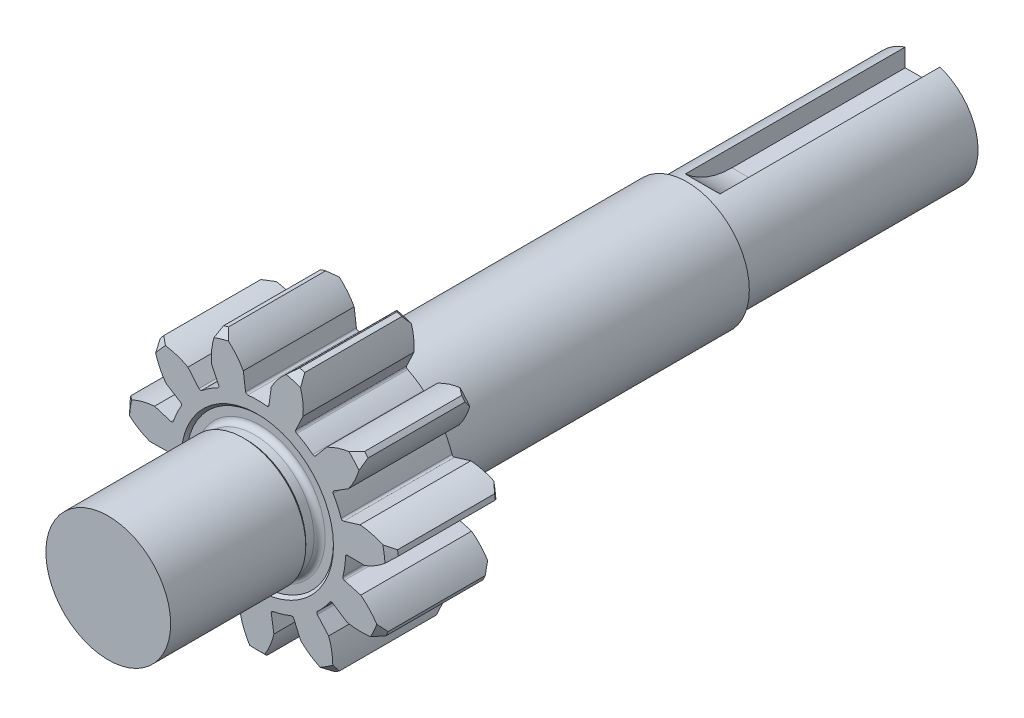
SolidWorks part; units mm, degrees
ref_plane "Middle plane" through (0, 0, 0) normal (0, 0, 1) x (1, 0, 0)
ref_plane "Top Plane" through (0, 0, 0) normal (0, 1, 0) x (1, 0, 0)
ref_plane "Right Plane" through (0, 0, 0) normal (1, 0, 0) x (0, 0, -1)
sketch "Spur gear" plane through (0, 0, 0) normal (0, 0, 1) x (1, 0, 0)
  line L0 (0, 0) -> (-2.3482, 16.3321) construction
  line L2 (-2.0154, 15.3734) -> (0, 0)
  line L3 (0, 0) -> (0, 52) construction
  line L4 (2.3482, 16.3321) -> (0, 0) construction
  line L6 (0, 0) -> (2.0154, 15.3734)
  circle A0 centre (0, 0) radius 15.5049
  circle A1 centre (0, 0) radius 12.75
  arc A2 (2.3482, 16.3321) -> (-2.3482, 16.3321) centre (0, 0) ccw
  circle A3 centre (0, 0) radius 19.5
  spline S0 degree 4 poles (0.7936, 14.8906) (0.7924, 14.9201) (0.7881, 14.9788) (0.7725, 15.0958) (0.7289, 15.316) (0.6484, 15.6067) (0.4539, 16.1447) (0.0492, 16.9597) (-0.6377, 17.9757) (-1.7913, 19.243) (-3.3499, 20.5096) (-5.2443, 21.6406) (-7.4338, 22.5657) (-9.7197, 23.2127) (-12.0632, 23.5974) (-14.5507, 23.7418) (-17.633, 23.5986) (-21.2621, 22.9576) (-25.3266, 21.6048) (-29.5547, 19.4226) (-33.4233, 16.6565) (-36.4497, 13.8025) (-38.7654, 11.0977) (-40.5023, 8.6952) (-41.7738, 6.6932) (-43.2134, 4.102) (-44.4514, 1.4058) (-45.4859, -1.3736) (-46.4831, -4.7889) (-47.0485, -7.396) (-47.4104, -9.7431) (-47.6077, -11.655) (-47.6802, -12.5487) (-47.7381, -13.4181) (-47.7759, -14.2391) (-47.8017, -14.99) (-47.8125, -16.0362) (-47.809, -16.7047) (-47.7875, -17.792) (-47.7473, -18.6332) (-47.688, -19.6577) (-47.6107, -20.5673) (-47.515, -21.548) (-47.4014, -22.4756) (-47.3026, -23.2033) (-47.2309, -23.6656) (-47.1936, -23.9061) knots 0 0 0 0 0 0.001401 0.002802 0.005604 0.010661 0.015718 0.02996 0.048734 0.068727 0.096889 0.125051 0.153212 0.181374 0.209535 0.237696 0.271429 0.327752 0.384075 0.440398 0.496721 0.553044 0.581206 0.609367 0.637529 0.66569 0.722013 0.750174 0.778336 0.834659 0.84874 0.86282 0.869861 0.876901 0.890982 0.900036 0.909091 0.920455 0.931818 0.943182 0.954545 0.965909 0.977273 0.988636 1 1 1 1 1 construction
  spline S1 degree 4 poles (-2.0154, 15.3734) (-2.1011, 15.5352) (-2.3813, 16.0225) (-2.9403, 16.8122) (-3.9842, 17.9417) (-5.4871, 19.1443) (-7.3108, 20.2145) (-9.4159, 21.0852) (-11.6114, 21.6888) (-13.8601, 22.0406) (-16.2451, 22.1609) (-19.1981, 22.0014) (-22.6715, 21.3607) (-26.557, 20.0349) (-30.5934, 17.9129) (-34.281, 15.2339) (-37.1607, 12.4768) (-39.3605, 9.8678) (-41.0077, 7.5528) (-42.2118, 5.6248) (-43.5728, 3.1311) (-44.7397, 0.5381) (-45.711, -2.1331) (-46.642, -5.4134) (-47.1651, -7.9161) (-47.4949, -10.1682) (-47.6701, -12.0019) (-47.7331, -12.8589) (-47.7823, -13.6926) (-47.8127, -14.4797) (-47.8319, -15.1995) (-47.8347, -16.2022) (-47.8265, -16.8429) (-47.798, -17.8848) (-47.7547, -18.6666) (-47.709, -19.3683) (-47.6743, -19.799) (-47.6569, -19.9982) knots 0.020881 0.020881 0.020881 0.020881 0.020881 0.02996 0.048734 0.068727 0.096889 0.125051 0.153212 0.181374 0.209535 0.237696 0.271429 0.327752 0.384075 0.440398 0.496721 0.553044 0.581206 0.609367 0.637529 0.66569 0.722013 0.750174 0.778336 0.834659 0.84874 0.86282 0.869861 0.876901 0.890982 0.900036 0.909091 0.920455 0.931818 0.943182 0.953189 0.953189 0.953189 0.953189 0.953189
  spline S2 degree 4 poles (-0.7936, 14.8906) (-0.7924, 14.9201) (-0.7881, 14.9788) (-0.7725, 15.0958) (-0.7289, 15.316) (-0.6484, 15.6067) (-0.4539, 16.1447) (-0.0492, 16.9597) (0.6377, 17.9757) (1.7913, 19.243) (3.3499, 20.5096) (5.2443, 21.6406) (7.4338, 22.5657) (9.7197, 23.2127) (12.0632, 23.5974) (14.5507, 23.7418) (17.633, 23.5986) (21.2621, 22.9576) (25.3266, 21.6048) (29.5547, 19.4226) (33.4233, 16.6565) (36.4497, 13.8025) (38.7654, 11.0977) (40.5023, 8.6952) (41.7738, 6.6932) (43.2134, 4.102) (44.4514, 1.4058) (45.4859, -1.3736) (46.4831, -4.7889) (47.0485, -7.396) (47.4104, -9.7431) (47.6077, -11.655) (47.6802, -12.5487) (47.7381, -13.4181) (47.7759, -14.2391) (47.8017, -14.99) (47.8125, -16.0362) (47.809, -16.7047) (47.7875, -17.792) (47.7473, -18.6332) (47.688, -19.6577) (47.6107, -20.5673) (47.515, -21.548) (47.4014, -22.4756) (47.3026, -23.2033) (47.2309, -23.6656) (47.1936, -23.9061) knots 0 0 0 0 0 0.001401 0.002802 0.005604 0.010661 0.015718 0.02996 0.048734 0.068727 0.096889 0.125051 0.153212 0.181374 0.209535 0.237696 0.271429 0.327752 0.384075 0.440398 0.496721 0.553044 0.581206 0.609367 0.637529 0.66569 0.722013 0.750174 0.778336 0.834659 0.84874 0.86282 0.869861 0.876901 0.890982 0.900036 0.909091 0.920455 0.931818 0.943182 0.954545 0.965909 0.977273 0.988636 1 1 1 1 1 construction
  spline S3 degree 4 poles (2.0154, 15.3734) (2.1011, 15.5352) (2.3813, 16.0225) (2.9403, 16.8122) (3.9842, 17.9417) (5.4871, 19.1443) (7.3108, 20.2145) (9.4159, 21.0852) (11.6114, 21.6888) (13.8601, 22.0406) (16.2451, 22.1609) (19.1981, 22.0014) (22.6715, 21.3607) (26.557, 20.0349) (30.5934, 17.9129) (34.281, 15.2339) (37.1607, 12.4768) (39.3605, 9.8678) (41.0077, 7.5528) (42.2118, 5.6248) (43.5728, 3.1311) (44.7397, 0.5381) (45.711, -2.1331) (46.642, -5.4134) (47.1651, -7.9161) (47.4949, -10.1682) (47.6701, -12.0019) (47.7331, -12.8589) (47.7823, -13.6926) (47.8127, -14.4797) (47.8319, -15.1995) (47.8347, -16.2022) (47.8265, -16.8429) (47.798, -17.8848) (47.7547, -18.6666) (47.709, -19.3683) (47.6743, -19.799) (47.6569, -19.9982) knots 0.020881 0.020881 0.020881 0.020881 0.020881 0.02996 0.048734 0.068727 0.096889 0.125051 0.153212 0.181374 0.209535 0.237696 0.271429 0.327752 0.384075 0.440398 0.496721 0.553044 0.581206 0.609367 0.637529 0.66569 0.722013 0.750174 0.778336 0.834659 0.84874 0.86282 0.869861 0.876901 0.890982 0.900036 0.909091 0.920455 0.931818 0.943182 0.953189 0.953189 0.953189 0.953189 0.953189
sketch "Circle" plane through (0, 0, 0) normal (0, 0, 1) x (1, 0, 0)
  circle A0 centre (0, 0) radius 19.5 construction
  circle A1 centre (0, 0) radius 19.5
extrude "Blank" add sketch "Circle" along normal mid plane 16
chamfer "Tooth chamfer" distance 1 angle 45 2 edges at (19.5, 0, -8) (19.5, 0, 8)
sketch "Tooth profile" plane through (0, 0, 0) normal (0, 0, 1) x (1, 0, 0)
  line L4 (0, 0) -> (2.0154, 15.3734) construction
  line L5 (-2.0154, 15.3734) -> (0, 0) construction
  line L6 (0, 0) -> (2.0154, 15.3734)
  line L7 (-2.0154, 15.3734) -> (0, 0)
  circle A4 centre (0, 0) radius 12.75 construction
  circle A5 centre (0, 0) radius 19.5 construction
  circle A6 centre (0, 0) radius 12.75
  circle A7 centre (0, 0) radius 19.5
  spline S1 degree 4 poles (999.7609, -51.6744) (36.065, -17.0379) (-0.5755, 0.4417) (-1.8205, 11.6607) (3.9842, 17.9417) (5.4871, 19.1443) (7.3108, 20.2145) (9.4159, 21.0852) (11.6114, 21.6888) (13.8601, 22.0406) (16.2451, 22.1609) (19.1981, 22.0014) (22.6715, 21.3607) (26.557, 20.0349) (30.5934, 17.9129) (34.281, 15.2339) (37.1607, 12.4768) (39.3605, 9.8678) (41.0077, 7.5528) (42.2118, 5.6248) (43.5728, 3.1311) (44.7397, 0.5381) (45.711, -2.1331) (46.642, -5.4134) (47.1651, -7.9161) (47.4949, -10.1682) (47.6701, -12.0019) (47.7331, -12.8589) (47.7823, -13.6926) (47.8127, -14.4797) (47.8319, -15.1995) (47.8347, -16.2022) (47.8265, -16.8429) (47.798, -17.8848) (47.5897, -21.6461) (46.8818, -29.7714) (46.3891, 13.6269) (33.8189, -1019.6941) knots -0.325788 -0.325788 -0.325788 -0.325788 -0.325788 0.02996 0.048734 0.068727 0.096889 0.125051 0.153212 0.181374 0.209535 0.237696 0.271429 0.327752 0.384075 0.440398 0.496721 0.553044 0.581206 0.609367 0.637529 0.66569 0.722013 0.750174 0.778336 0.834659 0.84874 0.86282 0.869861 0.876901 0.890982 0.900036 0.909091 0.920455 0.931818 0.943182 1.121242 1.121242 1.121242 1.121242 1.121242 only from (2.0154, 15.3734) to (47.6569, -19.9982) construction
  spline S3 degree 4 poles (-999.7609, -51.6744) (-36.065, -17.0379) (0.5755, 0.4417) (1.8205, 11.6607) (-3.9842, 17.9417) (-5.4871, 19.1443) (-7.3108, 20.2145) (-9.4159, 21.0852) (-11.6114, 21.6888) (-13.8601, 22.0406) (-16.2451, 22.1609) (-19.1981, 22.0014) (-22.6715, 21.3607) (-26.557, 20.0349) (-30.5934, 17.9129) (-34.281, 15.2339) (-37.1607, 12.4768) (-39.3605, 9.8678) (-41.0077, 7.5528) (-42.2118, 5.6248) (-43.5728, 3.1311) (-44.7397, 0.5381) (-45.711, -2.1331) (-46.642, -5.4134) (-47.1651, -7.9161) (-47.4949, -10.1682) (-47.6701, -12.0019) (-47.7331, -12.8589) (-47.7823, -13.6926) (-47.8127, -14.4797) (-47.8319, -15.1995) (-47.8347, -16.2022) (-47.8265, -16.8429) (-47.798, -17.8848) (-47.5897, -21.6461) (-46.8818, -29.7714) (-46.3891, 13.6269) (-33.8189, -1019.6941) knots -0.325788 -0.325788 -0.325788 -0.325788 -0.325788 0.02996 0.048734 0.068727 0.096889 0.125051 0.153212 0.181374 0.209535 0.237696 0.271429 0.327752 0.384075 0.440398 0.496721 0.553044 0.581206 0.609367 0.637529 0.66569 0.722013 0.750174 0.778336 0.834659 0.84874 0.86282 0.869861 0.876901 0.890982 0.900036 0.909091 0.920455 0.931818 0.943182 1.121242 1.121242 1.121242 1.121242 1.121242 only from (-2.0154, 15.3734) to (-47.6569, -19.9982) construction
  spline S4 degree 4 poles (2.0154, 15.3734) (2.1011, 15.5352) (2.3813, 16.0225) (2.9403, 16.8122) (3.9842, 17.9417) (5.4871, 19.1443) (7.3108, 20.2145) (9.4159, 21.0852) (11.6114, 21.6888) (13.8601, 22.0406) (16.2451, 22.1609) (19.1981, 22.0014) (22.6715, 21.3607) (26.557, 20.0349) (30.5934, 17.9129) (34.281, 15.2339) (37.1607, 12.4768) (39.3605, 9.8678) (41.0077, 7.5528) (42.2118, 5.6248) (43.5728, 3.1311) (44.7397, 0.5381) (45.711, -2.1331) (46.642, -5.4134) (47.1651, -7.9161) (47.4949, -10.1682) (47.6701, -12.0019) (47.7331, -12.8589) (47.7823, -13.6926) (47.8127, -14.4797) (47.8319, -15.1995) (47.8347, -16.2022) (47.8265, -16.8429) (47.798, -17.8848) (47.7547, -18.6666) (47.709, -19.3683) (47.6743, -19.799) (47.6569, -19.9982) knots 0.020881 0.020881 0.020881 0.020881 0.020881 0.02996 0.048734 0.068727 0.096889 0.125051 0.153212 0.181374 0.209535 0.237696 0.271429 0.327752 0.384075 0.440398 0.496721 0.553044 0.581206 0.609367 0.637529 0.66569 0.722013 0.750174 0.778336 0.834659 0.84874 0.86282 0.869861 0.876901 0.890982 0.900036 0.909091 0.920455 0.931818 0.943182 0.953189 0.953189 0.953189 0.953189 0.953189
  spline S5 degree 4 poles (-2.0154, 15.3734) (-2.1011, 15.5352) (-2.3813, 16.0225) (-2.9403, 16.8122) (-3.9842, 17.9417) (-5.4871, 19.1443) (-7.3108, 20.2145) (-9.4159, 21.0852) (-11.6114, 21.6888) (-13.8601, 22.0406) (-16.2451, 22.1609) (-19.1981, 22.0014) (-22.6715, 21.3607) (-26.557, 20.0349) (-30.5934, 17.9129) (-34.281, 15.2339) (-37.1607, 12.4768) (-39.3605, 9.8678) (-41.0077, 7.5528) (-42.2118, 5.6248) (-43.5728, 3.1311) (-44.7397, 0.5381) (-45.711, -2.1331) (-46.642, -5.4134) (-47.1651, -7.9161) (-47.4949, -10.1682) (-47.6701, -12.0019) (-47.7331, -12.8589) (-47.7823, -13.6926) (-47.8127, -14.4797) (-47.8319, -15.1995) (-47.8347, -16.2022) (-47.8265, -16.8429) (-47.798, -17.8848) (-47.7547, -18.6666) (-47.709, -19.3683) (-47.6743, -19.799) (-47.6569, -19.9982) knots 0.020881 0.020881 0.020881 0.020881 0.020881 0.02996 0.048734 0.068727 0.096889 0.125051 0.153212 0.181374 0.209535 0.237696 0.271429 0.327752 0.384075 0.440398 0.496721 0.553044 0.581206 0.609367 0.637529 0.66569 0.722013 0.750174 0.778336 0.834659 0.84874 0.86282 0.869861 0.876901 0.890982 0.900036 0.909091 0.920455 0.931818 0.943182 0.953189 0.953189 0.953189 0.953189 0.953189
extrude "Gear shaping" cut sketch "Tooth profile" against normal mid plane 16 contours S5 A6 S4 A7
fillet "Fillet1" [suppressed] radius 0.3
pattern_circular "CirPattern1" [suppressed] count 11 over 360
fillet "Fillet2" radius 0.3 2 edges at (1.6573, 12.6418, 0) (-1.6573, 12.6418, 0)
pattern_circular "CirPattern2" count 11 over 360 about axis through (0, 0, 8) along (0, 0, -1) of "Fillet2", "Gear shaping"
sketch "Pitch circle" plane through (0, 0, 0) normal (0, 0, 1) x (1, 0, 0)
  circle A0 centre (0, 0) radius 16.5 construction
  circle A1 centre (0, 0) radius 16.5 construction
sketch "Sketch1" plane through (0, 0, 8) normal (0, 0, 1) x (1, 0, 0)
  circle A0 centre (0, 0) radius 9
  dimension "D1" = 18
extrude "Boss-Extrude1" add sketch "Sketch1" along normal blind 21.5
sketch "Sketch2" plane through (0, 0, 29.5) normal (0, 0, 1) x (1, 0, 0)
  circle A0 centre (0, 0) radius 8
  dimension "D1" = 16
extrude "Boss-Extrude2" add sketch "Sketch2" along normal blind 34 from offset 117.5 separate body offset against normal yes
sketch "Sketch3" plane through (0, 0, -54) normal (0, 0, 1) x (1, 0, 0)
  circle A0 centre (0, 0) radius 9
  dimension "D1" = 18
extrude "Boss-Extrude3" add sketch "Sketch3" along normal up to surface (46 mm away) up to face at (0, 0, -8)
sketch "Sketch4" plane through (0, 0, 0) normal (1, 0, 0) x (0, 0, -1)
  line L0 (88, 5) -> (63, 5)
  line L1 (88, -8) -> (88, 8) construction
  line L2 (55.8586, 8) -> (88, 8)
  line L3 (88, 8) -> (88, 5)
  line L4 (54, -8) -> (88, -8) construction
  arc A0 (63, 5) -> (55.8586, 8) centre (63, 15) cw
  dimension "D1" = 25
  dimension "D2" = 10
  dimension "D3" = 25
  dimension "D4" = 13
extrude "Cut-Extrude1" cut sketch "Sketch4" against normal mid plane 5
sketch "Sketch5" plane through (0, 0, 0) normal (1, 0, 0) x (0, 0, -1)
  line L4 (8, 11) -> (7.6, 10.6)
  line L5 (8, 9) -> (7.6, 8.6) construction
  line L6 (8, 9) -> (10, 9)
  line L7 (7.6, 8.6) -> (9.6, 8.6)
  line L8 (10, 9) -> (9.6, 8.6)
  line L9 (7.6, 8.6) -> (7.6, 10.6)
  line L10 (8, 9) -> (8, 11)
  line L11 (0, 0) -> (0, 9.5985) construction
  line L12 (0, 16.5) -> (0, -16.5) construction
  line L14 (-8, 9) -> (-7.6, 8.6) construction
  line L15 (-8, 9) -> (-8, 11)
  line L16 (-7.6, 8.6) -> (-7.6, 10.6)
  line L17 (-10, 9) -> (-9.6, 8.6)
  line L18 (-7.6, 8.6) -> (-9.6, 8.6)
  line L19 (-8, 9) -> (-10, 9)
  line L20 (-8, 11) -> (-7.6, 10.6)
  line L21 (0, 0) -> (11.406, 0) construction
  dimension "D1" = 45
  dimension "D2" = 2
  dimension "D3" = 0.4
revolve "Cut-Revolve1" cut sketch "Sketch5" angle 360 about L21
fillet "Fillet3" radius 0.8 2 edges at (8.6, 0, 7.6) (8.6, 0, -7.6)
equation "\"m\"= 3'模数"
equation "\"z\"= 11'齿数"
equation "\"a\"= 20'压力角（常见为20°）"
equation "\"B\"= 16'齿宽"
equation "\"C1\"= 1'轮齿倒角（若设为0，则无倒角）"
equation "\"x\"= 0'变位系数（不懂勿动）"
equation "\"ha\"= 1'齿顶高系数（不懂勿动）"
equation "\"c\"= 0.25'顶隙系数（不懂勿动）"
equation "\"基圆直径@Spur gear\"= \"m\" * \"z\" * cos ( \"a\" )"
equation "\"齿根圆@Spur gear\" = \"m\" * ( \"z\" - 2 * ( \"ha\" - \"x\" + \"c\" ) )"
equation "\"分度圆@Spur gear\"=\"m\" * \"z\""
equation "\"齿顶圆@Spur gear\" = \"m\" * ( \"z\" + 2 * ( \"ha\" + \"x\" ) )"
equation "\"R\"= 0.3'齿根圆角"
equation "\"D1\"= \"R\""
equation "\"D1@Blank\" = \"B\""
equation "\"D1@Tooth chamfer\" = IIF ( \"C1\" > 0 , \"C1\" , 0.001 )"
equation "\"轮齿倒角\"= IIF ( \"C1\" > 0 , \"unsuppressed\" , \"suppressed\" )"
equation "\"D1@Gear shaping\" = \"B\""
equation "\"D1@CirPattern1\" = \"z\""
equation "\"D1@Spur gear\"= \"m\" * ( pi / 2 ) - 2 * \"m\" * tan ( \"a\" ) * \"x\"'作者：机械菌-"
equation "\"D1@Fillet1\"=\"R\""
equation "\"圆角1\" = IIF ( \"m\" * ( \"z\" - 2 * ( \"ha\" - \"x\" + \"c\" ) ) > \"m\" * \"z\" * cos ( \"a\" ) , \"unsuppressed\" , \"suppressed\" )"
equation "\"圆周阵列1\"= IIF ( \"m\" * ( \"z\" - 2 * ( \"ha\" - \"x\" + \"c\" ) ) > \"m\" * \"z\" * cos ( \"a\" ) , \"unsuppressed\" , \"suppressed\" )"
equation "\"D1@Fillet2\"=\"R\""
equation "\"D1@CirPattern2\" = \"z\""
equation "\"圆角2\" = IIF ( \"m\" * ( \"z\" - 2 * ( \"ha\" - \"x\" + \"c\" ) ) < \"m\" * \"z\" * cos ( \"a\" ) , \"unsuppressed\" , \"suppressed\" )"
equation "\"圆周阵列2\"= IIF ( \"m\" *  ( \"z\" - 2 *  ( \"ha\" - \"x\" + \"c\" )  )  < \"m\" * \"z\" * cos ( \"a\" )  ,  unsuppressed  ,  suppressed  ) "
